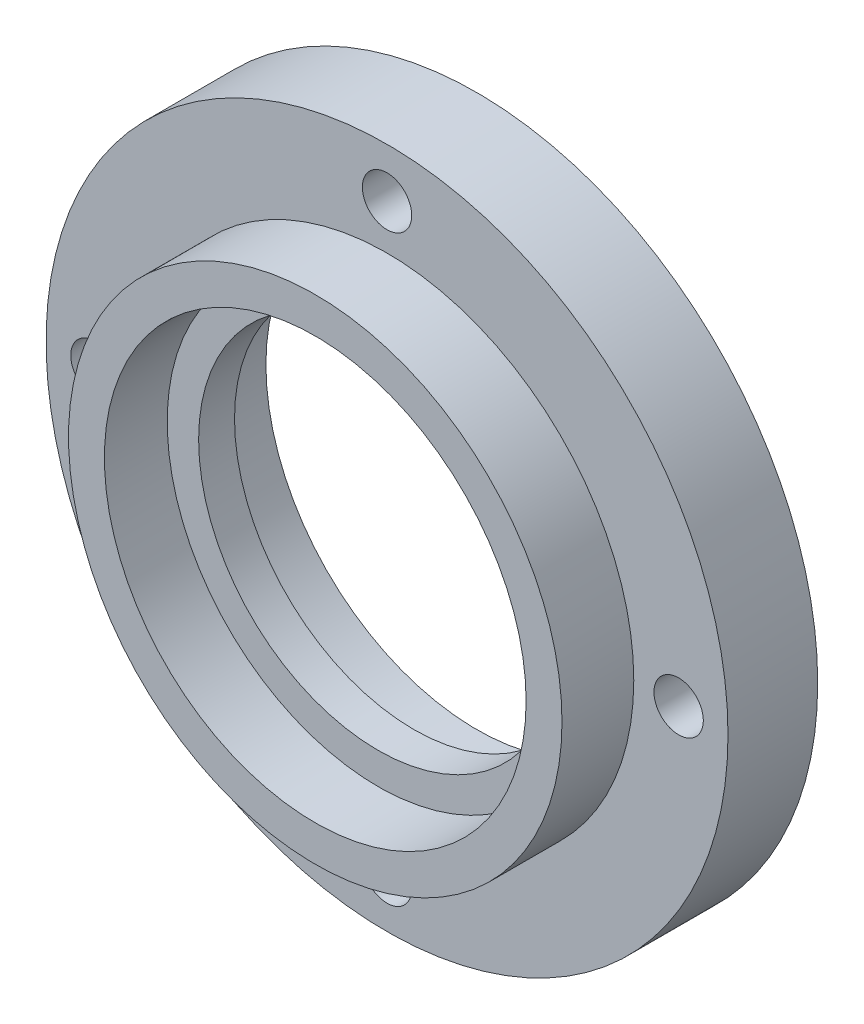
SolidWorks part; units mm, degrees
material "S45C"
ref_plane "Front Plane" through (0, 0, 0) normal (0, 0, 1) x (1, 0, 0)
ref_plane "Top Plane" through (0, 0, 0) normal (0, 1, 0) x (1, 0, 0)
ref_plane "Right Plane" through (0, 0, 0) normal (1, 0, 0) x (0, 0, -1)
sketch "Sketch1" plane through (0, 0, 0) normal (0, 0, 1) x (1, 0, 0)
  circle A0 centre (0, 0) radius 38
  dimension "D1" = 76
extrude "Boss-Extrude1" add sketch "Sketch1" along normal blind 10
sketch "Sketch2" plane through (0, 0, 10) normal (0, 0, 1) x (1, 0, 0)
  circle A0 centre (0, 0) radius 27.5
  dimension "D1" = 55
extrude "Boss-Extrude2" add sketch "Sketch2" along normal blind 8
sketch "Sketch3" plane through (0, 0, 18) normal (0, 0, 1) x (1, 0, 0)
  circle A0 centre (0, 0) radius 23.5
  dimension "D1" = 47
extrude "Cut-Extrude1" cut sketch "Sketch3" against normal blind 7
sketch "Sketch4" plane through (0, 0, 0) normal (0, 0, -1) x (-1, 0, 0)
  circle A0 centre (0, 0) radius 23.5
  dimension "D1" = 47
extrude "Cut-Extrude2" cut sketch "Sketch4" against normal blind 7
sketch "Sketch6" plane through (0, 0, 18) normal (0, 0, 1) x (1, 0, 0)
  circle A0 centre (0, 0) radius 20
  dimension "D1" = 40
extrude "Cut-Extrude3" cut sketch "Sketch6" against normal through all
hole_wizard "CBORE for M5 Hex Socket Head Cap Screw1" positions "Sketch7" profile "Sketch8" counterbore size "M5" standard "ISO" end condition through all
sketch "Sketch7" plane through (0, 0, 0) normal (0, 0, -1) x (-1, 0, 0)
  line L3 (0, 32.5) -> (-32.5, 0) construction
  line L4 (-32.5, 0) -> (0, -32.5) construction
  line L5 (0, -32.5) -> (32.5, 0) construction
  line L6 (32.5, 0) -> (0, 32.5) construction
  circle A0 centre (0, 0) radius 32.5 construction
  point P0 (0, 32.5)
  point P10 (-32.5, 0)
  point P11 (0, -32.5)
  point P12 (32.5, 0)
  dimension "D1" = 65
sketch "Sketch8" plane through (0, 32.5, 0) normal (1, 0, 0) x (0, 1, 0)
  line L0 (0, 0) -> (0, 18)
  line L1 (0, 18) -> (2.75, 18)
  line L3 (2.75, 18) -> (2.75, 5.4)
  line L4 (2.75, 5.4) -> (5, 5.4)
  line L5 (5, 5.4) -> (5, 0)
  line L7 (5, 0) -> (0, 0)
  line L11 (0, -6.35) -> (0, 107.95) construction
  dimension "通孔孔直径" = 5.5
  dimension "通孔孔深度" = 18
  dimension "柱形沉头孔直径" = 10
  dimension "柱形沉头孔深度" = 5.4
